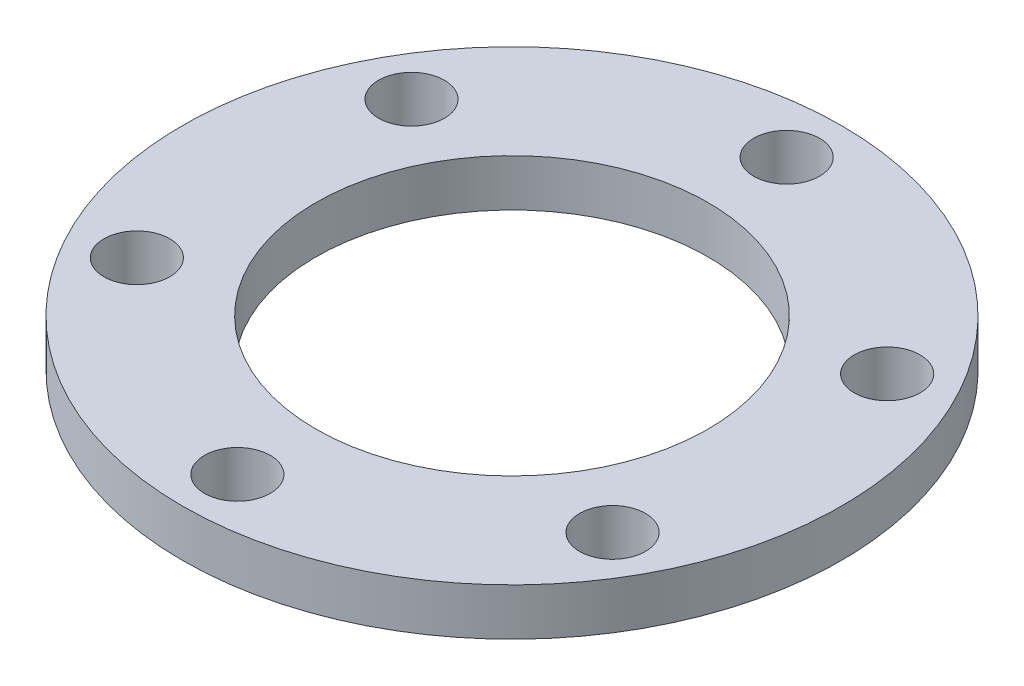
SolidWorks part; units mm, degrees
material "哈碳纤"
ref_plane "前视基准面" through (0, 0, 0) normal (0, 0, 1) x (1, 0, 0)
ref_plane "上视基准面" through (0, 0, 0) normal (0, 1, 0) x (1, 0, 0)
ref_plane "右视基准面" through (0, 0, 0) normal (1, 0, 0) x (0, 0, -1)
other "Configuration Table"
sketch "草图1" plane through (0, 0, 0) normal (0, 1, 0) x (1, 0, 0)
  circle A0 centre (0, 0) radius 12.5
  circle A2 centre (0, 0) radius 17.5 construction
  circle A3 centre (0, 0) radius 21
  circle A4 centre (0, 17.5) radius 2.1
  circle A5 centre (15.1554, 8.75) radius 2.1
  circle A6 centre (15.1554, -8.75) radius 2.1
  circle A7 centre (0, -17.5) radius 2.1
  circle A8 centre (-15.1554, -8.75) radius 2.1
  circle A9 centre (-15.1554, 8.75) radius 2.1
  point P7 (-17.61, -9.3995)
  point P8 (0, 0)
  point P19 (0, 0)
  dimension "D1" = 25
  dimension "D2" = 35
  dimension "D3" = 42
  dimension "D4" = 4.2
  dimension "D5" = 6
extrude "凸台-拉伸1" add sketch "草图1" along normal blind 3
